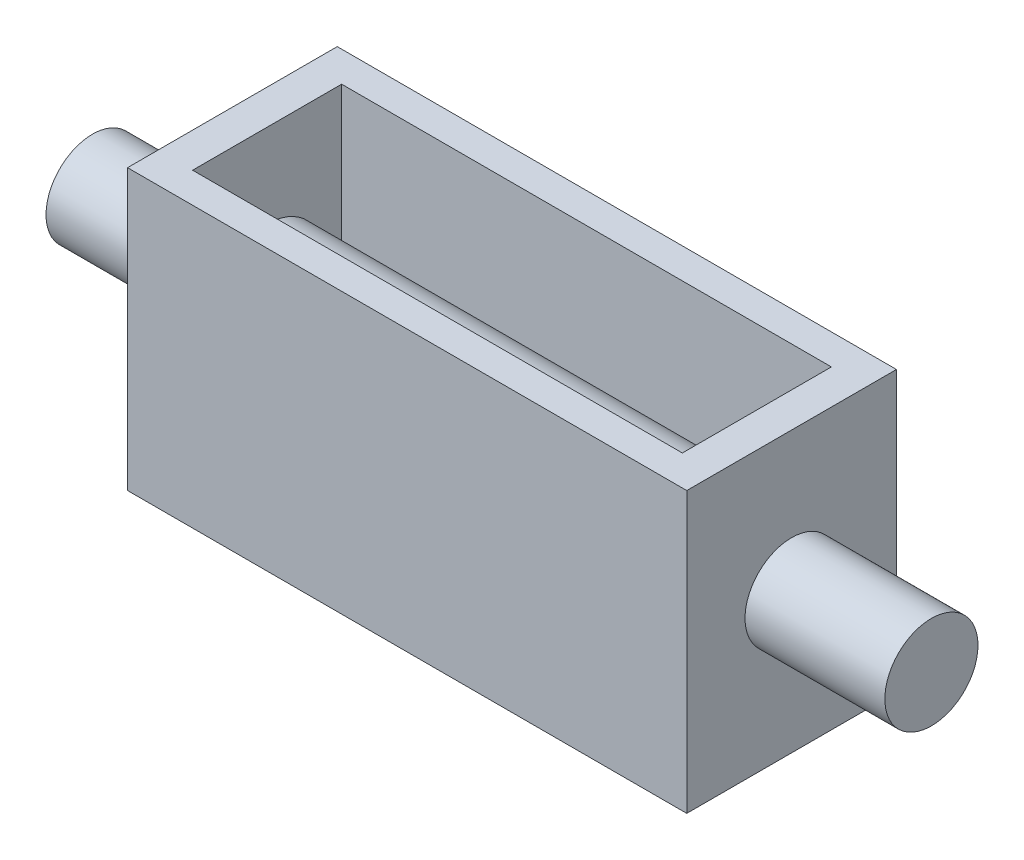
SolidWorks part; units mm, degrees
ref_plane "Front Plane" through (0, 0, 0) normal (0, 0, 1) x (1, 0, 0)
ref_plane "Top Plane" through (0, 0, 0) normal (0, 1, 0) x (1, 0, 0)
ref_plane "Right Plane" through (0, 0, 0) normal (1, 0, 0) x (0, 0, -1)
sketch "Sketch1" plane through (0, 0, 0) normal (0, 1, 0) x (1, 0, 0)
  line L1 (-20, 7.5) -> (20, 7.5)
  line L2 (-20, 7.5) -> (-20, -7.5)
  line L3 (-20, -7.5) -> (20, -7.5)
  line L4 (20, 7.5) -> (20, -7.5)
  line L5 (-20, 7.5) -> (20, -7.5) construction
  line L6 (-20, -7.5) -> (20, 7.5) construction
  point P0 (0, 0)
  dimension "D1" = 40
  dimension "D2" = 15
extrude "Boss-Extrude1" add sketch "Sketch1" along normal blind 20
sketch "Sketch2" plane through (0, 20, 0) normal (0, 1, 0) x (1, 0, 0)
  line L1 (-17.5161, -5.3302) -> (17.5161, -5.3302)
  line L2 (-17.5161, -5.3302) -> (-17.5161, 5.3302)
  line L3 (-17.5161, 5.3302) -> (17.5161, 5.3302)
  line L4 (17.5161, -5.3302) -> (17.5161, 5.3302)
  line L5 (-17.5161, -5.3302) -> (17.5161, 5.3302) construction
  line L6 (-17.5161, 5.3302) -> (17.5161, -5.3302) construction
  point P0 (0, 0)
extrude "Cut-Extrude1" cut sketch "Sketch2" against normal blind 10
sketch "Sketch3" plane through (-17.5161, 0, 0) normal (1, 0, 0) x (0, 0, -1)
  line L0 (5.3302, 20) -> (-5.3302, 20) construction
  circle A0 centre (0, 10) radius 4
  dimension "D1" = 10
  dimension "D2" = 8
extrude "Boss-Extrude2" add sketch "Sketch3" along normal up to surface (35.0321 mm away) up to face at (17.5161, 15, 0)
sketch "Sketch4" plane through (-20, 0, 0) normal (-1, 0, 0) x (0, 0, 1)
  circle A0 centre (0, 10) radius 3.3323
extrude "Boss-Extrude3" add sketch "Sketch4" along normal blind 10
sketch "Sketch5" plane through (20, 0, 0) normal (1, 0, 0) x (0, 0, -1)
  circle A1 centre (0, 10) radius 3.3323
  circle A2 centre (0, 10) radius 3.3323
  dimension "D1" = 0
extrude "Boss-Extrude4" add sketch "Sketch5" along normal blind 10
scale "Scale1" bodies to scale 105 scale about origin uniform scaling yes scale factor 0.7
